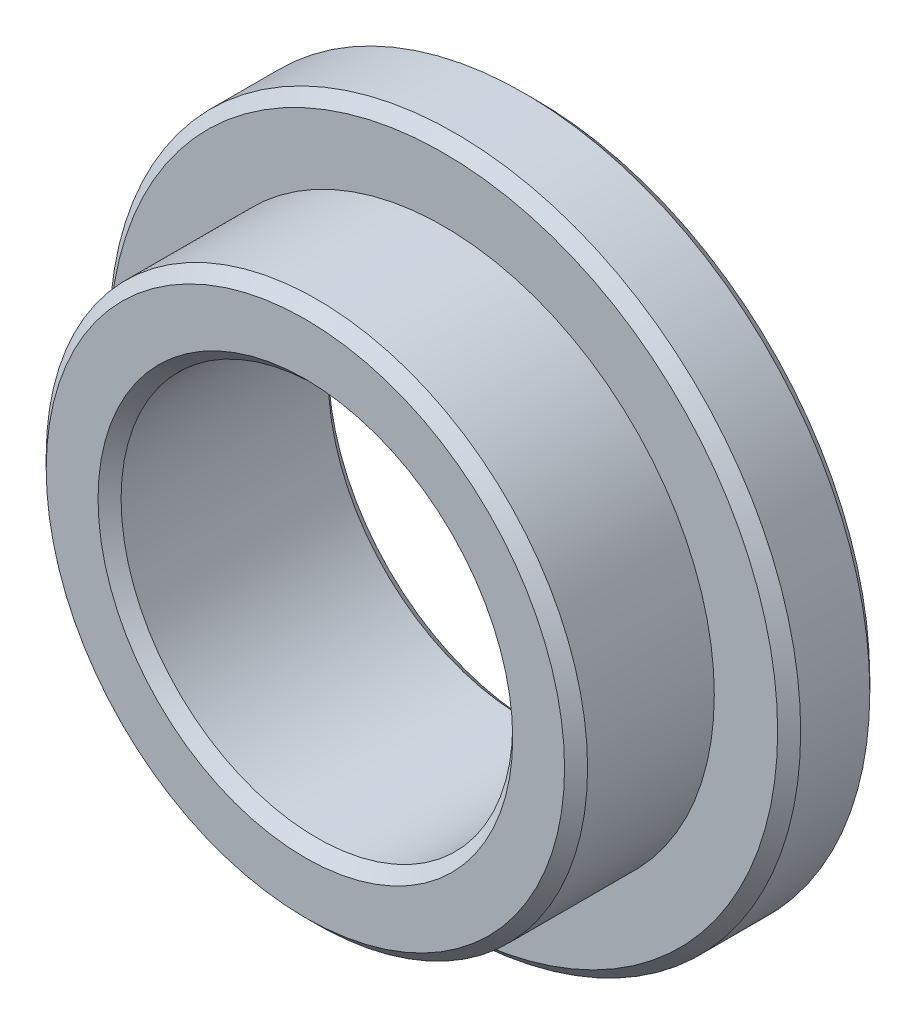
from build123d import *

# Parameters (mm, degrees)
SKETCH1_R           = 15
BOSS_EXTRUDE1_DEPTH = 4
SKETCH2_R           = 11.75
BOSS_EXTRUDE2_DEPTH = 6
SKETCH3_R           = 8.5
CUT_EXTRUDE1_DEPTH  = 20
CHAMFER1_SIZE       = 0.5
CHAMFER2_SIZE       = 0.5


with BuildPart() as part:
    # Sketch1 → Boss-Extrude1 (new body)
    with BuildSketch(Plane.XY):
        Circle(SKETCH1_R)
    extrude(amount=BOSS_EXTRUDE1_DEPTH)

    # Sketch2 → Boss-Extrude2 (add)
    with BuildSketch(Plane.XY.offset(4)):
        Circle(SKETCH2_R)
    extrude(amount=BOSS_EXTRUDE2_DEPTH)

    # Sketch3 → Cut-Extrude1 (cut)
    with BuildSketch(Plane(origin=(0, 0, 0), x_dir=(-1, 0, 0), z_dir=(0, 0, -1))):
        Circle(SKETCH3_R)
    extrude(amount=-CUT_EXTRUDE1_DEPTH, mode=Mode.SUBTRACT)

    # Chamfer1
    chamfer1_edges = [part.edges().sort_by_distance(p)[0] for p in [
        (8.5, 0, 10),
        (8.5, 0, 0),
    ]]
    chamfer(chamfer1_edges, length=CHAMFER1_SIZE)

    # Chamfer2
    chamfer2_edges = [part.edges().sort_by_distance(p)[0] for p in [
        (-15, 0, 0),
        (-15, 0, 4),
        (-11.75, 0, 10),
    ]]
    chamfer(chamfer2_edges, length=CHAMFER2_SIZE)


solid = part.part
